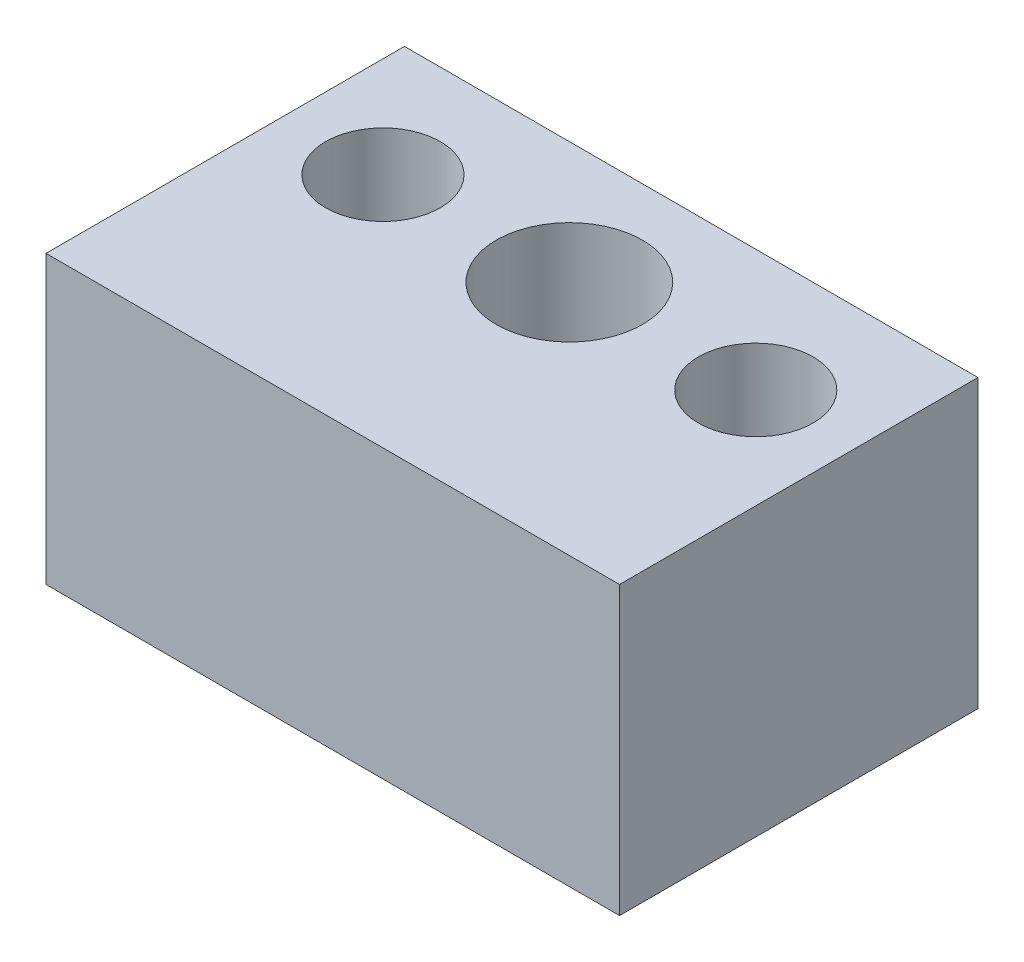
from build123d import *

# Parameters (mm, degrees)
SKETCH_1_W              = 40
SKETCH_1_H              = 20
EXTRUDE_1_DEPTH         = 8.5
CUT_EXTRUDE_1_REACH     = 31.534
SKETCH_2_R              = 4
CUT_EXTRUDE_2_REACH     = 31.534
SKETCH_3_R              = 4
SKETCH_6_W              = 40
SKETCH_6_H              = 20
EXTRUDE_3_DEPTH         = 8
HOLE_WIZARD_M12_1_D     = 10.2
HOLE_WIZARD_M12_1_DEPTH = 20


with BuildPart() as part:
    # 草图1 → 凸台-拉伸1 (new, symmetric)
    with BuildSketch(Plane.XY):
        Rectangle(SKETCH_1_W, SKETCH_1_H)
    extrude(amount=EXTRUDE_1_DEPTH, both=True)

    # 草图2 → 切除-拉伸1 (cut, up to next)
    with BuildSketch(Plane(origin=(0, 10, 0), x_dir=(1, 0, 0), z_dir=(0, 1, 0)), mode=Mode.PRIVATE) as cut_extrude_1_sk1:
        with Locations(Location((-13, 0, 0), (0, 0, 270))):
            Circle(SKETCH_2_R)
    cut_extrude_1_tool1 = extrude(cut_extrude_1_sk1.sketch, amount=-CUT_EXTRUDE_1_REACH, mode=Mode.PRIVATE) & part.part
    # 草图2 → 切除-拉伸1 (cut, up to next)
    with BuildSketch(Plane(origin=(0, 10, 0), x_dir=(1, 0, 0), z_dir=(0, 1, 0)), mode=Mode.PRIVATE) as cut_extrude_1_sk2:
        with Locations(Location((13, 0, 0), (0, 0, 270))):
            Circle(SKETCH_2_R)
    cut_extrude_1_tool2 = extrude(cut_extrude_1_sk2.sketch, amount=-CUT_EXTRUDE_1_REACH, mode=Mode.PRIVATE) & part.part
    add(cut_extrude_1_tool1.solids().sort_by_distance((-13, 10, 0))[0], mode=Mode.SUBTRACT)
    add(cut_extrude_1_tool2.solids().sort_by_distance((13, 10, 0))[0], mode=Mode.SUBTRACT)

    # 草图3 → 切除-拉伸2 (cut, up to next)
    with BuildSketch(Plane.XZ.offset(10), mode=Mode.PRIVATE) as cut_extrude_2_sk1:
        with Locations(Location((0, 0, 0), (0, 0, 270))):
            Circle(SKETCH_3_R)
    cut_extrude_2_tool1 = extrude(cut_extrude_2_sk1.sketch, amount=-CUT_EXTRUDE_2_REACH, mode=Mode.PRIVATE) & part.part
    add(cut_extrude_2_tool1.solids().sort_by_distance((0, -10, 0))[0], mode=Mode.SUBTRACT)

    # 草图6 → 凸台-拉伸3 (add)
    with BuildSketch(Plane.XY.offset(8.5)):
        Rectangle(SKETCH_6_W, SKETCH_6_H)
    extrude(amount=EXTRUDE_3_DEPTH)

    # M12 螺纹孔1
    with Locations(Plane.ZX.offset(10)):
        with Locations((0, 0)):
            Hole(HOLE_WIZARD_M12_1_D / 2, depth=HOLE_WIZARD_M12_1_DEPTH)


solid = part.part
